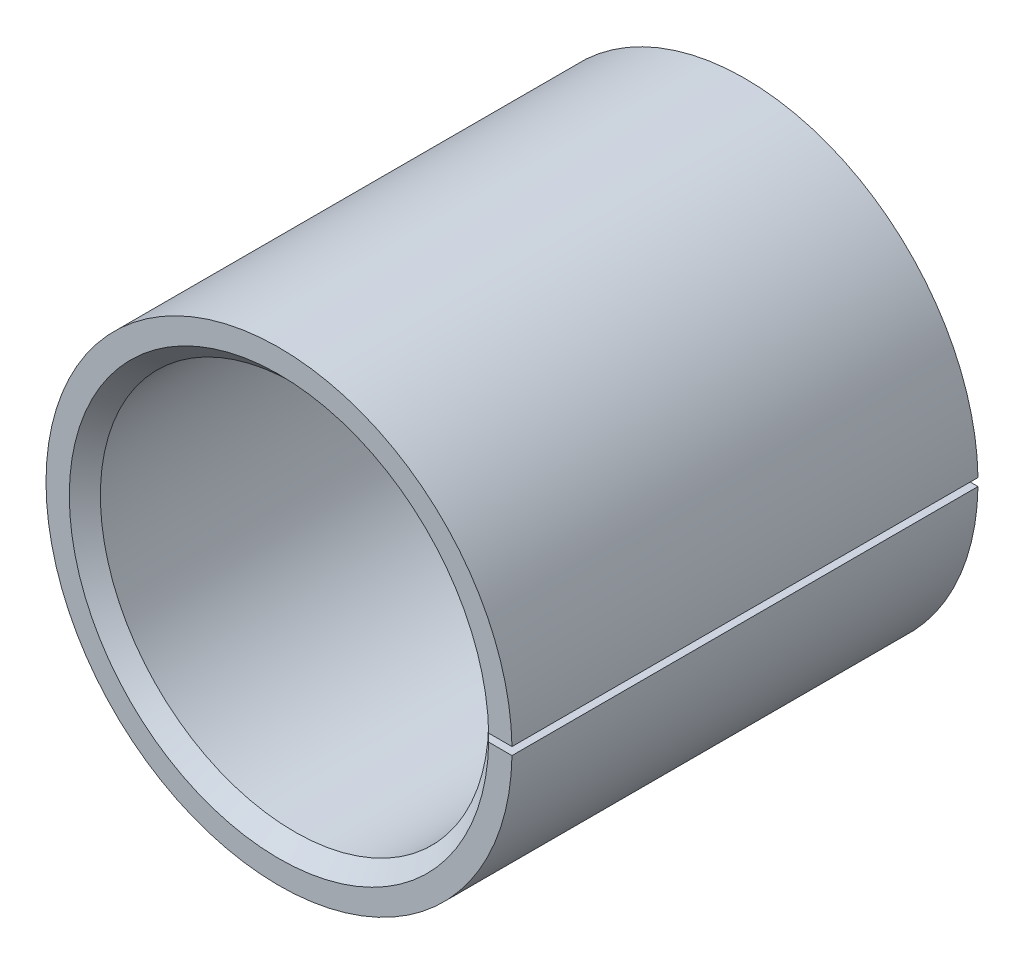
SolidWorks part; units mm, degrees
ref_plane "Front Plane" through (0, 0, 0) normal (0, 0, 1) x (1, 0, 0)
ref_plane "Top Plane" through (0, 0, 0) normal (0, 1, 0) x (1, 0, 0)
ref_plane "Right Plane" through (0, 0, 0) normal (1, 0, 0) x (0, 0, -1)
other "Configuration Table"
sketch "Sketch1" plane through (0, 0, 0) normal (0, 0, 1) x (1, 0, 0)
  circle A0 centre (0, 0) radius 2.5
  circle A1 centre (0, 0) radius 3
  dimension "D1" = 6
  dimension "D2" = 5
extrude "Boss-Extrude1" add sketch "Sketch1" along normal blind 6
chamfer "Chamfer1" distance 0.2 angle 45 2 edges at (2.5, 0, 0) (2.5, 0, 6)
sketch "Sketch2" plane through (0, 0, 6) normal (0, 0, 1) x (1, 0, 0)
  line L0 (0, 0) -> (3, 0) construction
  line L1 (0.6418, 0.05) -> (5.3582, 0.05)
  line L2 (0.6418, 0.05) -> (0.6418, -0.05)
  line L3 (0.6418, -0.05) -> (5.3582, -0.05)
  line L4 (5.3582, 0.05) -> (5.3582, -0.05)
  line L5 (0.6418, 0.05) -> (5.3582, -0.05) construction
  line L6 (0.6418, -0.05) -> (5.3582, 0.05) construction
  circle A0 centre (0, 0) radius 3 construction
  point P0 (3, 0)
  dimension "D1" = 0.1
extrude "Cut-Extrude1" cut sketch "Sketch2" against normal blind 6
